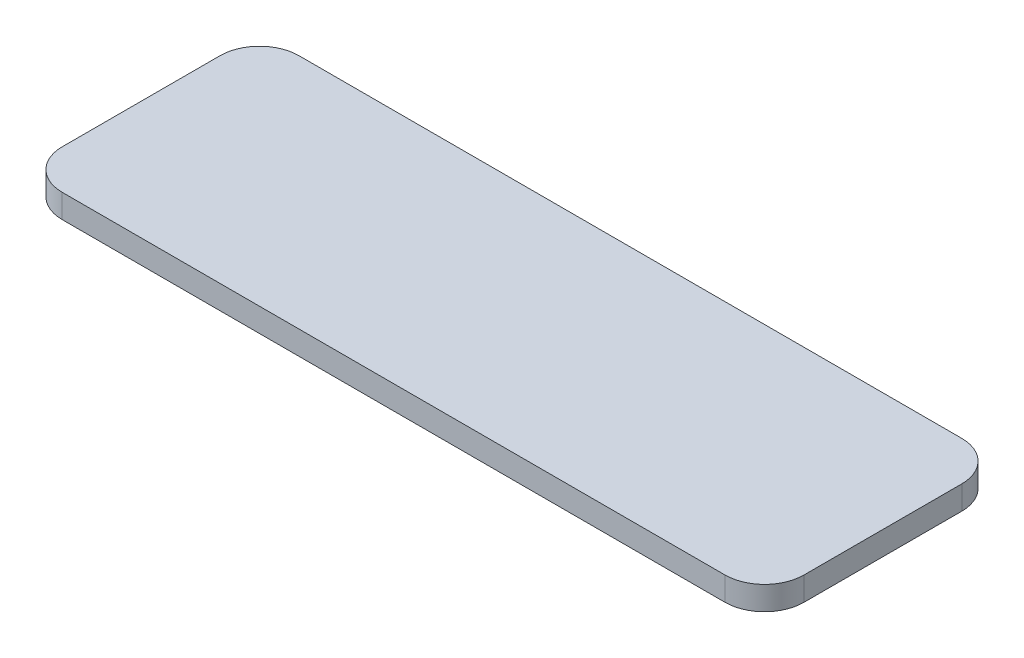
from build123d import *

# Parameters (mm, degrees)
SKETCH1_W           = 94
SKETCH1_H           = 30
BOSS_EXTRUDE1_DEPTH = 3
FILLET1_R           = 5


with BuildPart() as part:
    # Sketch1 → Boss-Extrude1 (new body)
    with BuildSketch(Plane(origin=(0, 0, 0), x_dir=(1, 0, 0), z_dir=(0, 1, 0))):
        Rectangle(SKETCH1_W, SKETCH1_H)
    extrude(amount=BOSS_EXTRUDE1_DEPTH)

    # Fillet1
    fillet1_edges = [part.edges().sort_by_distance(p)[0] for p in [
        (47, 1.5, 15),
        (-47, 1.5, 15),
        (-47, 1.5, -15),
        (47, 1.5, -15),
    ]]
    fillet(fillet1_edges, radius=FILLET1_R)


solid = part.part
